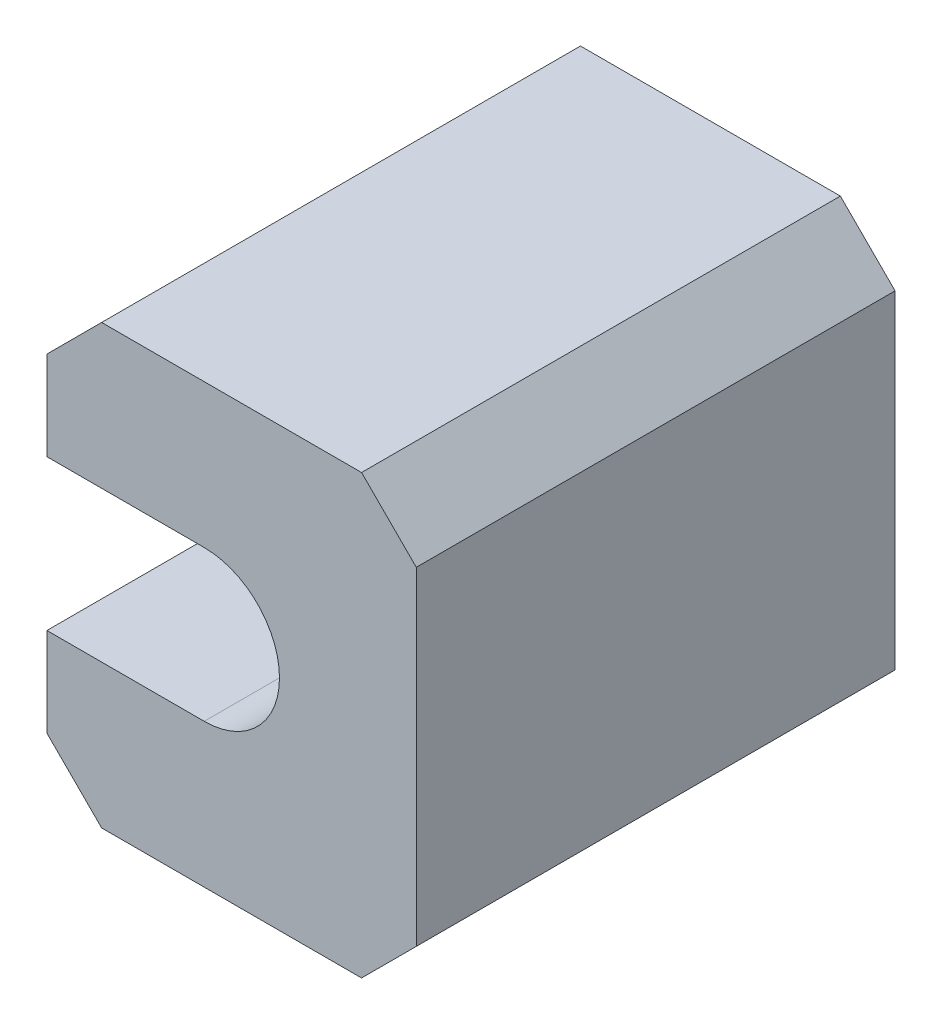
from build123d import *

# Parameters (mm, degrees)
BOSS_EXTRUDE1_DEPTH = 70


with BuildPart() as part:
    # Sketch1 → Boss-Extrude1 (new body)
    with BuildSketch(Plane.XY):
        with BuildLine():
            Line((0, 8), (0, 56))
            Line((0, 56), (-8, 64))
            Line((-8, 64), (-46, 64))
            Line((-46, 64), (-54, 56))
            Line((-54, 56), (-54, 43))
            Line((-54, 43), (-31, 43))
            ThreePointArc((-31, 43), (-20, 32), (-31, 21))
            Line((-31, 21), (-54, 21))
            Line((-54, 21), (-54, 8))
            Line((-54, 8), (-46, 0))
            Line((-46, 0), (-8, 0))
            Line((-8, 0), (0, 8))
        make_face()
    extrude(amount=BOSS_EXTRUDE1_DEPTH)


solid = part.part
